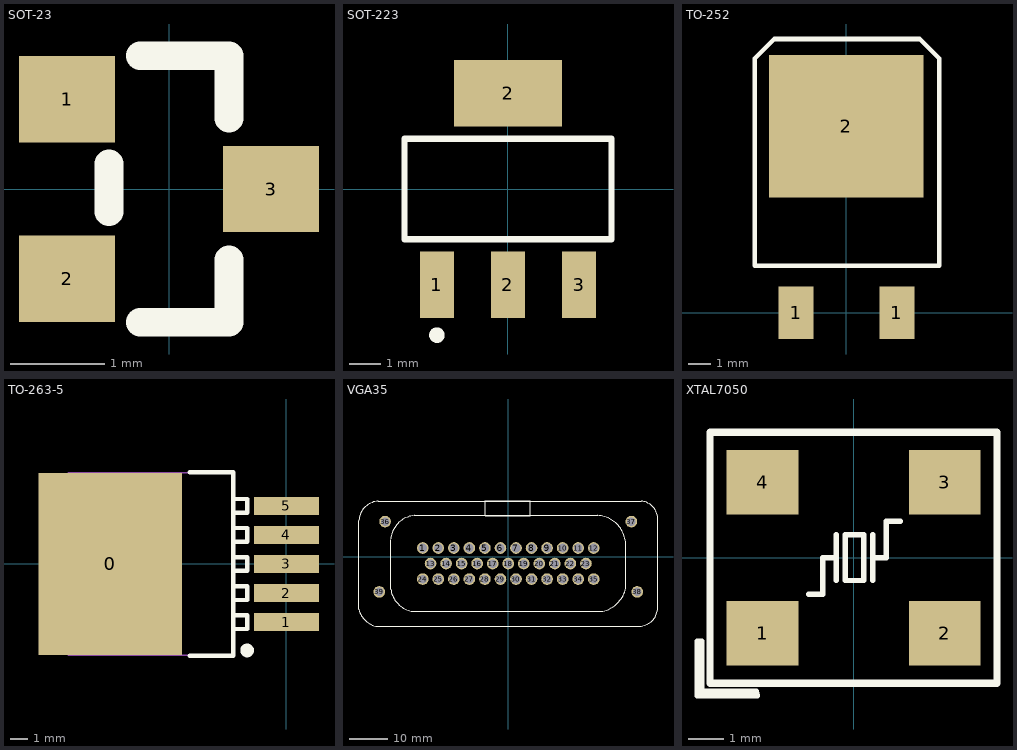
[diagram p0: the footprints below, top view; thin cyan lines are the x and y axes]
# Altium footprint library MISC82155.PcbLib: 38 footprints (part 3 of 3)
Each footprint in its own frame and in the unit in brackets; x right, y up, seen from the top. Pads: shape width x height; smd on the part's side, far side on the other; paste and mask are expansions set on the pad; w line width, h text height; cw(c..) or ccw(c..) is an arc to the next point about the centre after c.

## SOT-23 [mil]
height 374.02
pads (3):
  rect 40x36 smd: 1(-42.5,37.4) 2(-42.5,-37.4) 3(42.5,0)
Top Overlay:
  lines w12: -25,-9.5 -25,10.5 ; -12,-55.5 25,-55.5 25,-29.5 ; -12,55.5 25,55.5 25,29.5
3D body: height 39.37, standoff -0.79, extent -47,-56.98 50.48,57.98

## SOT-223 [mm]
height 3.98
pads (4):
  rect 1.1x2.15 smd: 1(-2.3,-3.1) 2(0,-3.1) 3(2.3,-3.1)
  rect 3.5x2.15 smd: 2(0,3.1)
Top Overlay:
  circle w0.25: c-2.3,-4.725 r0.125
  lines w0.2: -3.35,-1.625 3.35,-1.625 3.35,1.625 -3.35,1.625 -3.35,-1.625
3D body: height 1.8, standoff 0, extent -3.15,-3.3 3.15,3.3

## TO-252 [mm] "DPAK"
height 3.98
pads (3):
  rect 1.524x2.28 smd: 1(-2.2,0) 1(2.2,0)
  rect 6.74x6.23 smd: 2(0,8.14)
Top Overlay:
  lines w0.203: -4,2.05 4.05,2.05 4.05,11.1 3.2,11.95 -3.15,11.95 -4,11.1 -4,2.05
3D body: height 2.2, standoff 0, extent -3.24,-0.5 3.26,10.5

## TO-263-5 [mm]
pads (6):
  rect 8.4x10.65 smd: 0(-10.3,0)
  rect 3.8x1.05 smd: 1(0,-3.4) 2(0,-1.7) 3(0,0) 4(0,1.7) 5(0,3.4)
Top Overlay:
  circle w0.4: c-2.3,-5.05 r0.2
  lines w0.254: -5.65,-5.35 -3.1,-5.35 -3.1,5.35 -5.65,5.35 ; -3.1,-3 -2.3,-3 -2.3,-3.8 -3,-3.8 ; -3.1,-1.3 -2.3,-1.3 -2.3,-2.1 -3,-2.1 ; -3.1,0.4 -2.3,0.4 -2.3,-0.4 -3,-0.4 ; -3.1,2.1 -2.3,2.1 -2.3,1.3 -3,1.3 ; -3.1,3.8 -2.3,3.8 -2.3,3 -3,3
Mechanical 13:
  lines w0.1: -12.75,-5.325 -3.1,-5.325 -3.1,5.325 -12.75,5.325 -12.75,-5.325

## VGA35 [mm]
height 9.5
pads (39):
  round 3 hole 2.2: 1(-22,2.25) 2(-18,2.25) 3(-14,2.25) 4(-10,2.25) 5(-6,2.25) 6(-2,2.25) 7(2,2.25) 8(6,2.25) 9(10,2.25) 10(14,2.25) 11(18,2.25) 12(22,2.25) 13(-20,-1.75) 14(-16,-1.75) 15(-12,-1.75) 16(-8,-1.75) 17(-4,-1.75) 18(0,-1.75) 19(4,-1.75) 20(8,-1.75) 21(12,-1.75) 22(16,-1.75) 23(20,-1.75) 24(-22,-5.75) 25(-18,-5.75) 26(-14,-5.75) 27(-10,-5.75) 28(-6,-5.75) 29(-2,-5.75) 30(2,-5.75) 31(6,-5.75) 32(10,-5.75) 33(14,-5.75) 34(18,-5.75) 35(22,-5.75) 36(-31.7,9.05) 37(31.7,9.05) 38(33.2,-9.05) 39(-33.2,-9.05)
Top Overlay:
  lines w0.3: -38.45,-13.567 -38.45,9.333 ; -38.451,9.38 cw(c-33.073,8.948) -33.506,14.325 34.218,14.326 ; -38.449,-13.569 ccw(c-32.521,-11.937) -34.154,-17.865 ; -34.152,-17.865 34.292,-17.865 ; -30.256,4.602 cw(c-23.428,3.812) -24.218,10.639 ; -30.24,-8.348 -30.24,4.425 ; -30.239,-8.355 ccw(c-23.556,-7.38) -24.52,-14.064 ; -24.524,-14.063 24.348,-14.063 ; -24.215,10.64 22.995,10.64 ; 22.991,10.64 cw(c22.561,2.948) 30.252,3.392 ; 24.341,-14.065 ccw(c22.376,-6.187) 30.251,-8.165 ; 30.252,-8.158 30.252,3.382 ; 34.216,14.326 cw(c33.843,9.688) 38.479,10.069 ; 34.285,-17.866 ccw(c33.431,-12.817) 38.48,-13.68 ; 38.48,-13.677 38.48,10.064 ; -5.952,10.605 5.636,10.605 5.636,14.359 -5.952,14.359 -5.952,10.605

## XTAL7050 [mm]
height 9.5
pads (4):
  rect 2x1.8 smd: 1(-2.54,-2.1) 2(2.54,-2.1) 3(2.54,2.1) 4(-2.54,2.1)
Top Overlay:
  lines w0.152: -1.245,-1.016 -0.864,-1.016 -0.864,0 -0.483,0 ; -0.483,-0.635 -0.483,0.635 ; 0.533,-0.635 0.533,0.635 ; 0.533,0 0.914,0 0.914,1.016 1.295,1.016 ; -4.367,-3.849 -2.69,-3.849 -2.716,-3.722 -4.24,-3.722 -4.24,-2.325 -4.367,-2.325 -4.367,-3.849 ; -0.229,-0.635 -0.229,0.635 0.279,0.635 0.279,-0.635 -0.229,-0.635
  lines w0.2: -4,-3.5 4,-3.5 4,3.5 -4,3.5 -4,-3.5